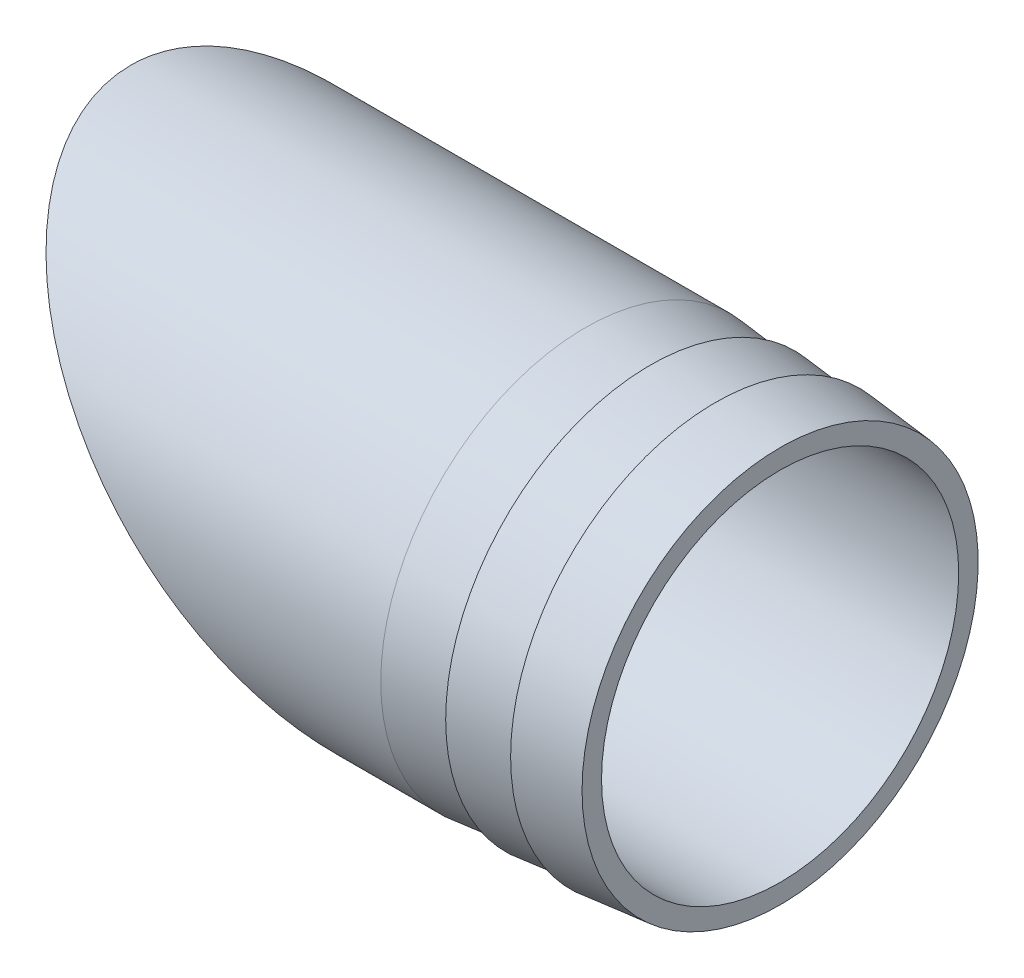
SolidWorks part; units mm, degrees
material "Q235"
ref_plane "Front Plane" through (0, 0, 0) normal (0, 0, 1) x (1, 0, 0)
ref_plane "Top Plane" through (0, 0, 0) normal (0, 1, 0) x (1, 0, 0)
ref_plane "Right Plane" through (0, 0, 0) normal (1, 0, 0) x (0, 0, -1)
sketch "Sketch1" plane through (0, 0, 0) normal (0, 0, 1) x (1, 0, 0)
  line L0 (0, 27.5) -> (0, 31.5)
  line L1 (0, 31.5) -> (70, 31.5)
  line L2 (70, 31.5) -> (80, 30.5)
  line L3 (80, 30.5) -> (80, 31.5)
  line L4 (80, 31.5) -> (90, 30.5)
  line L5 (90, 30.5) -> (90, 31.5)
  line L6 (90, 31.5) -> (100, 30.5)
  line L9 (100, 27.5) -> (0, 27.5)
  line L10 (0, 0) -> (17.4583, 0) construction
  line L11 (100, 30.5) -> (100, 27.5)
  dimension "D1" = 1
  dimension "D2" = 31.5
  dimension "D3" = 4
  dimension "D4" = 10
  dimension "D5" = 70
  dimension "D6" = 100
revolve "Revolve1" add sketch "Sketch1" angle 360 about L10
sketch "Sketch2" plane through (0, 0, 0) normal (0, 0, 1) x (1, 0, 0)
  line L0 (0, 31.5) -> (96.3337, -64.8337)
  line L1 (0, 31.5) -> (0, -31.5) construction
  dimension "D1" = 45
extrude "Cut-Extrude1" cut sketch "Sketch2" against normal through all both and the other way through all flip side to cut
